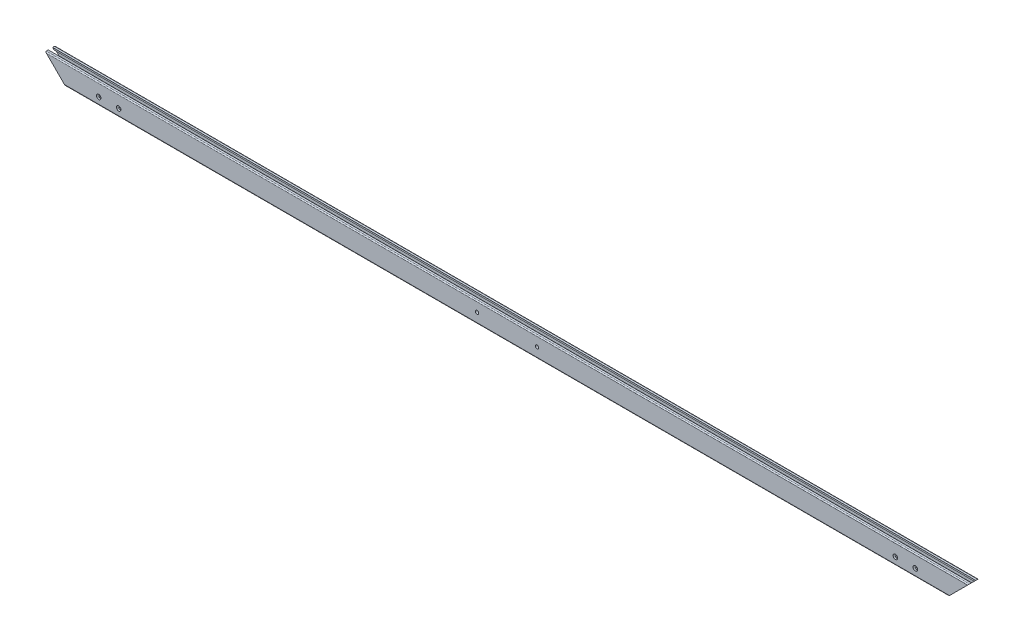
SolidWorks part; units mm, degrees
ref_plane "前视" through (0, 0, 0) normal (0, 0, 1) x (1, 0, 0)
ref_plane "上视" through (0, 0, 0) normal (0, 1, 0) x (1, 0, 0)
ref_plane "右视" through (0, 0, 0) normal (1, 0, 0) x (0, 0, -1)
sketch3d "3D草图1"
  line L0 (-693, 0, 0) -> (693, 0, 0)
  dimension "D1" = 1386
other "结构构件1"
ref_plane "基准面1" through (-693, 0, 0) normal (1, 0, 0) x (0, 0, -1)
sketch "Sketch11" plane through (-693, 0, 0) normal (1, 0, 0) x (0, 0, -1)
  line L1 (0, 16.311) -> (0, -16.311) construction
  line L2 (0, 0) -> (9.513, 0) construction
  line L3 (-6, -15) -> (-3.25, -15)
  line L4 (-7.5, -13.5) -> (-7.5, 13.5)
  line L5 (-6, 15) -> (-3.25, 15)
  line L6 (7.5, -13.5) -> (7.5, 13.5)
  line L17 (3.25, 15) -> (6, 15)
  line L20 (-5, 12.7) -> (-5, 7)
  line L21 (-3.25, 12.7) -> (-5, 12.7)
  line L24 (5, 12.7) -> (5, 7)
  line L25 (3.25, 12.7) -> (5, 12.7)
  line L26 (-3.25, 15) -> (-3.25, 12.7)
  line L27 (3.25, 15) -> (3.25, 12.7)
  line L40 (5, -12.7) -> (5, -7)
  line L41 (3.25, -12.7) -> (5, -12.7)
  line L44 (-5, -12.7) -> (-5, -7)
  line L45 (-3.25, -12.7) -> (-5, -12.7)
  line L47 (3.25, -15) -> (3.25, -12.7)
  line L48 (-3.25, -15) -> (-3.25, -12.7)
  line L49 (3.25, -15) -> (6, -15)
  arc A0 (-6, -15) -> (-7.5, -13.5) centre (-6, -13.5) cw
  arc A1 (6, -15) -> (7.5, -13.5) centre (6, -13.5) ccw
  arc A2 (6, 15) -> (7.5, 13.5) centre (6, 13.5) cw
  arc A3 (-7.5, 13.5) -> (-6, 15) centre (-6, 13.5) cw
  circle A4 centre (0, 0) radius 2.5
  arc A5 (-5, 7) -> (5, 7) centre (0, 10.3166) ccw
  arc A6 (-5, -7) -> (5, -7) centre (0, -10.3166) cw
  point P4 (0, 0)
  point P21 (0, 0)
  point P44 (-7.5, 15)
  point P45 (7.5, 15)
  point P46 (7.5, -15)
  point P47 (-7.5, -15)
  point P48 (0, -15)
  point P49 (0, 15)
  dimension "D1" = 30
  dimension "D2" = 15
  dimension "D3" = 1.5
  dimension "D4" = 5
  dimension "D5" = 6.5
  dimension "D6" = 6
  dimension "D7" = 8
  dimension "D8" = 10
  dimension "D9" = 2.3
sketch "草图4" plane through (0, 0, 7.5) normal (0, 0, 1) x (1, 0, 0)
  line L0 (-693, 15) -> (-663, -15)
  line L1 (693, -15) -> (-693, -15) construction
  line L2 (0, 0) -> (0, -85.0329) construction
  line L3 (-663, -15) -> (-693, -15)
  line L4 (-693, -15) -> (-693, 15)
  line L5 (693, -15) -> (693, 15)
  line L6 (663, -15) -> (693, -15)
  line L7 (693, 15) -> (663, -15)
extrude "切除-拉伸1" cut sketch "草图4" against normal through all
hole_wizard "M8 螺纹孔1" positions "草图6" profile "草图7" tap size "M8" standard "Iso" end condition through all
sketch "草图6" plane through (0, 0, 7.5) normal (0, 0, 1) x (1, 0, 0)
  line L0 (0, 0) -> (0, -60.6345) construction
  line L2 (693, 15) -> (-693, 15) construction
  point P0 (-613, -4)
  point P2 (-583, -4)
  point P9 (583, -4)
  point P10 (613, -4)
  dimension "D1" = 30
  dimension "D2" = 19
  dimension "D3" = 80
sketch "草图7" plane through (-613, -4, 7.5) normal (1, 0, 0) x (0, -1, 0)
  line L0 (0, 0) -> (0, 15)
  line L1 (0, 15) -> (3.4, 15)
  line L2 (3.4, 15) -> (3.4, 0)
  line L5 (3.4, 0) -> (0, 0)
  line L11 (0, -6.35) -> (0, 107.95) construction
  dimension "通孔螺纹孔钻头直径" = 6.8
  dimension "通孔螺纹孔钻头深度" = 15
cosmetic thread "孔螺蚊线1" parameters "D2"=8
cosmetic thread "孔螺蚊线2" parameters "D2"=8
cosmetic thread "孔螺蚊线3" parameters "D2"=8
cosmetic thread "孔螺蚊线4" parameters "D2"=8
hole_wizard "M6 螺纹孔1" positions "草图10" profile "草图9" tap size "M6" standard "Iso"
sketch "草图10" plane through (0, 0, 7.5) normal (0, 0, 1) x (1, 0, 0)
  line L0 (0, 0) -> (0, -25.2696) construction
  point P0 (-45, 0)
  point P2 (45, 0)
  dimension "D1" = 90
sketch "草图9" plane through (-45, 0, 7.5) normal (1, 0, 0) x (0, -1, 0)
  line L0 (0, 0) -> (0, 18.5022)
  line L1 (0, 18.5022) -> (2.5, 17)
  line L2 (2.5, 17) -> (2.5, 0)
  line L5 (2.5, 0) -> (0, 0)
  line L10 (0, 18.5022) -> (-2.5, 17) construction
  line L11 (0, -6.35) -> (0, 107.95) construction
  dimension "螺纹孔钻头直径" = 5
  dimension "螺纹孔钻头深度" = 17
  dimension "导头角度" = 118
cosmetic thread "孔螺蚊线5" parameters "D1"=12, "D2"=6
cosmetic thread "孔螺蚊线6" parameters "D1"=12, "D2"=6
